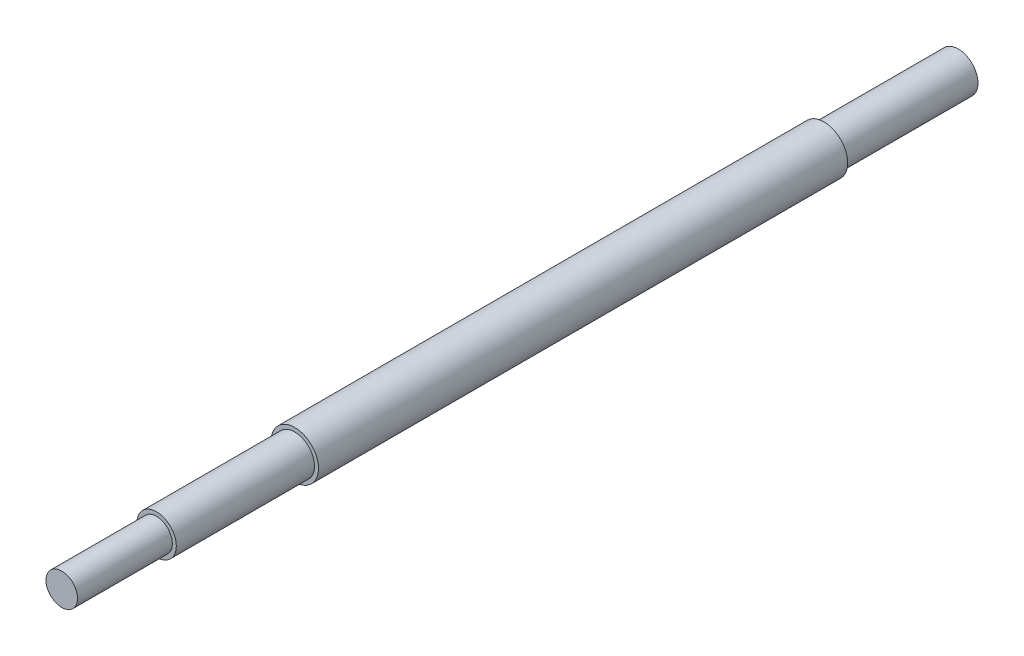
SolidWorks part; units mm, degrees
ref_plane "Front Plane" through (0, 0, 0) normal (0, 0, 1) x (1, 0, 0)
ref_plane "Top Plane" through (0, 0, 0) normal (0, 1, 0) x (1, 0, 0)
ref_plane "Right Plane" through (0, 0, 0) normal (1, 0, 0) x (0, 0, -1)
sketch "Sketch1" plane through (0, 0, 0) normal (0, 0, 1) x (1, 0, 0)
  circle A0 centre (0, 0) radius 2.5
extrude "Boss-Extrude1" add sketch "Sketch1" along normal blind 17
sketch "Sketch2" plane through (0, 0, 17) normal (0, 0, 1) x (1, 0, 0)
  circle A0 centre (0, 0) radius 3
extrude "Boss-Extrude2" add sketch "Sketch2" along normal blind 67
sketch "Sketch3" plane through (0, 0, 84) normal (0, 0, 1) x (1, 0, 0)
  circle A0 centre (0, 0) radius 2.5
extrude "Boss-Extrude3" add sketch "Sketch3" along normal blind 17.5
sketch "Sketch4" plane through (0, 0, 101.5) normal (0, 0, 1) x (1, 0, 0)
  circle A0 centre (0, 0) radius 2
extrude "Boss-Extrude4" add sketch "Sketch4" along normal blind 12
